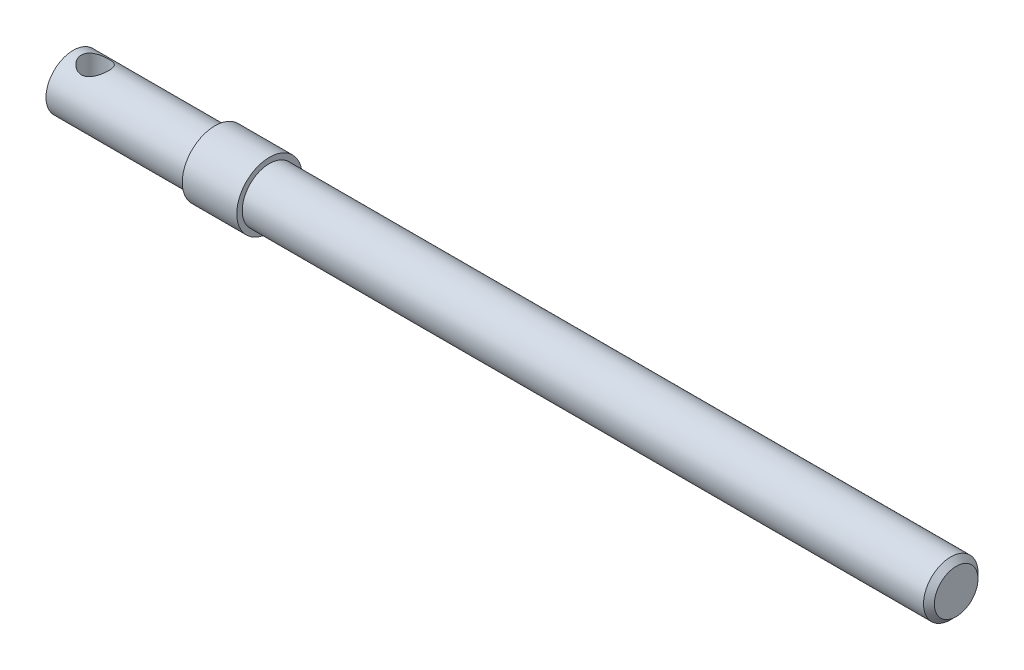
SolidWorks part; units mm, degrees
ref_plane "Front Plane" through (0, 0, 0) normal (0, 0, 1) x (1, 0, 0)
ref_plane "Top Plane" through (0, 0, 0) normal (0, 1, 0) x (1, 0, 0)
ref_plane "Right Plane" through (0, 0, 0) normal (1, 0, 0) x (0, 0, -1)
other "Configuration Table"
ref_plane "Plane1" through (0, 0, 0) normal (0, 0, -1) x (-1, 0, 0)
sketch "Sketch1" plane through (0, 0, 0) normal (0, 0, -1) x (-1, 0, 0)
  line L0 (-18, 3) -> (-18, 0)
  line L1 (-18, 0) -> (-13, 0)
  line L2 (-13, 0) -> (-13, 3)
  line L3 (-13, 3) -> (-18, 3)
  line L4 (-18, 0) -> (-13, 0) construction
revolve "Revolve1" add sketch "Sketch1" angle 360 about L4
sketch "Sketch2" plane through (13, 0, 0) normal (-1, 0, 0) x (0, 0, 1)
  circle A0 centre (0, 0) radius 2.5
extrude "Boss-Extrude1" add sketch "Sketch2" along normal blind 13
sketch "Sketch3" plane through (18, 0, 0) normal (1, 0, 0) x (0, 0, -1)
  circle A0 centre (0, 0) radius 2.5
extrude "Boss-Extrude2" add sketch "Sketch3" along normal blind 63
hole_wizard "Ø2.5 (2.5) Diameter Hole1" positions "3DSketch1" profile "Sketch4" hole size "Ø2.5" standard "ANSI Metric"
sketch3d "3DSketch1"
  point P0 (2, -2.5, 0)
sketch "Sketch4" plane through (2, -2.5, 0) normal (1, 0, 0) x (0, 0, -1)
  line L0 (0, 0) -> (0, 5.5)
  line L1 (0, 5.5) -> (1.25, 5.5)
  line L2 (1.25, 5.5) -> (1.25, 0)
  line L5 (1.25, 0) -> (0, 0)
  line L11 (0, -6.35) -> (0, 107.95) construction
  dimension "通孔孔直径" = 2.5
  dimension "通孔孔深度" = 5.5
chamfer "Chamfer1" distance 0.5 angle 45 1 edges at (81, 0, -2.5)
